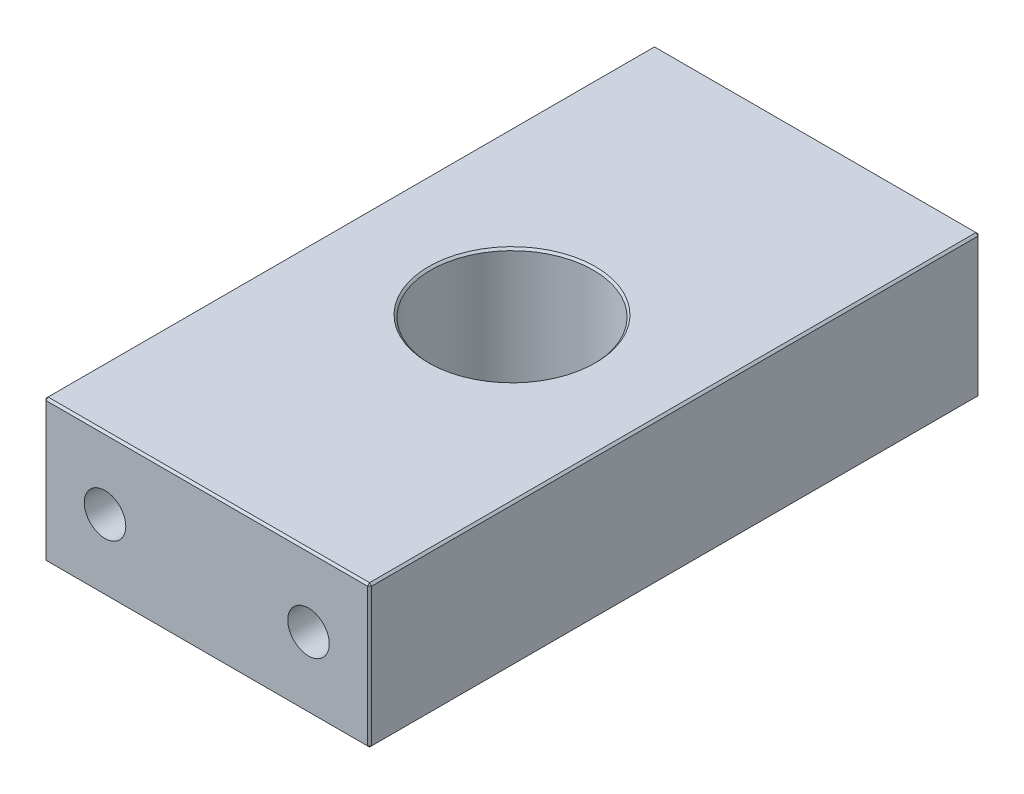
from build123d import *

# Parameters (mm, degrees)
SKETCH_1_W              = 80
SKETCH_1_H              = 150
SKETCH_1_R              = 20
EXTRUDE_1_DEPTH         = 35
CHAMFER_1_SIZE          = 0.5
HOLE_WIZARD_M12_1_D     = 10.2
HOLE_WIZARD_M12_1_DEPTH = 29.25
HOLE_WIZARD_M12_1_TIP   = 3.064389157
HOLE_WIZARD_M12_2_D     = 10.2
HOLE_WIZARD_M12_2_DEPTH = 29.25
HOLE_WIZARD_M12_2_TIP   = 3.064389157


with BuildPart() as part:
    # 草图1 → 凸台-拉伸1 (new body)
    with BuildSketch(Plane(origin=(0, 0, 0), x_dir=(1, 0, 0), z_dir=(0, 1, 0))):
        Rectangle(SKETCH_1_W, SKETCH_1_H)
        with Locations(Location((0, 0, 0), (0, 0, 270))):
            Circle(SKETCH_1_R, mode=Mode.SUBTRACT)
    extrude(amount=EXTRUDE_1_DEPTH)

    # 倒角1
    chamfer_1_edges = [part.edges().sort_by_distance(p)[0] for p in [
        (-40, 35, 0),
        (0, 0, -20),
        (0, 35, -20),
        (0, 35, 75),
        (40, 35, 0),
        (0, 0, 75),
        (-40, 0, 0),
        (0, 0, -75),
        (40, 0, 0),
        (0, 35, -75),
        (40, 17.5, 75),
        (-40, 17.5, 75),
        (-40, 17.5, -75),
        (40, 17.5, -75),
    ]]
    chamfer(chamfer_1_edges, length=CHAMFER_1_SIZE)

    # M12 螺纹孔1
    with Locations(Plane.XY.offset(75)):
        with Locations((25, 17.5), (-25, 17.5)):
            Hole(HOLE_WIZARD_M12_1_D / 2, depth=HOLE_WIZARD_M12_1_DEPTH)
            with Locations((0, 0, -(HOLE_WIZARD_M12_1_DEPTH + HOLE_WIZARD_M12_1_TIP / 2))):  # 118° drill point
                Cone(0, HOLE_WIZARD_M12_1_D / 2, HOLE_WIZARD_M12_1_TIP, mode=Mode.SUBTRACT)

    # M12 螺纹孔2
    with Locations(Plane(origin=(0, 0, -75), x_dir=(-1, 0, 0), z_dir=(0, 0, -1))):
        with Locations((-25, 17.5), (25, 17.5)):
            Hole(HOLE_WIZARD_M12_2_D / 2, depth=HOLE_WIZARD_M12_2_DEPTH)
            with Locations((0, 0, -(HOLE_WIZARD_M12_2_DEPTH + HOLE_WIZARD_M12_2_TIP / 2))):  # 118° drill point
                Cone(0, HOLE_WIZARD_M12_2_D / 2, HOLE_WIZARD_M12_2_TIP, mode=Mode.SUBTRACT)


solid = part.part
